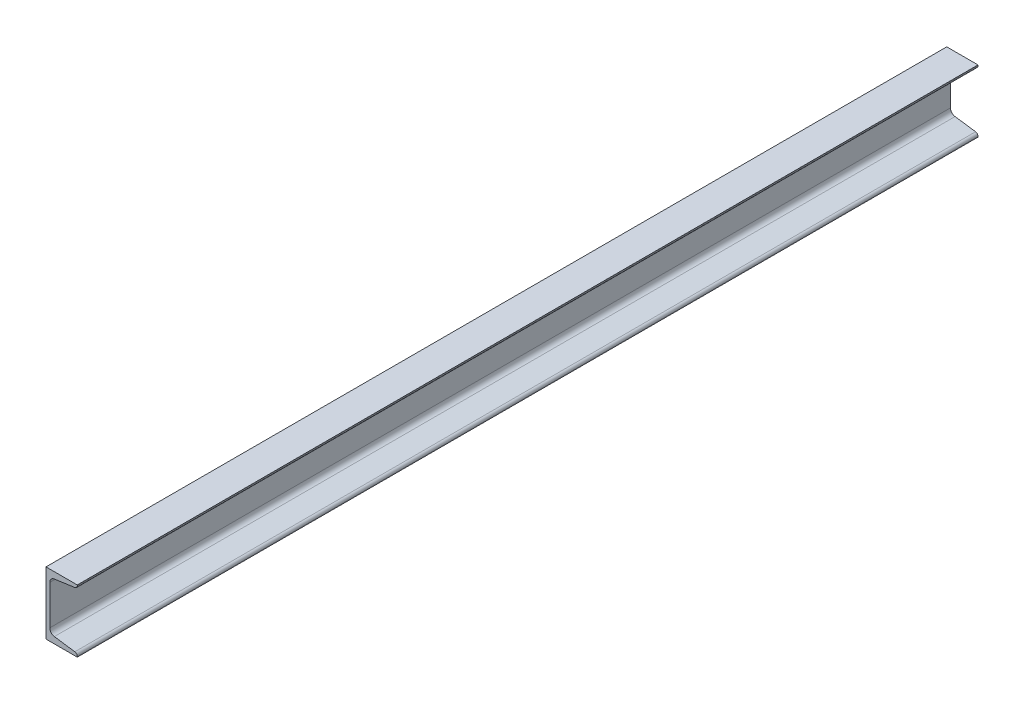
from build123d import *

# Parameters (mm, degrees)
BOSS_EXTRUDE1_DEPTH = 1440
SKETCH2_R           = 8.5
CUT_EXTRUDE1_DEPTH  = 1440


with BuildPart() as part:
    # Sketch1 → Boss-Extrude1 (new body)
    with BuildSketch(Plane.XY):
        with BuildLine():
            Line((0, 0), (-50, 0))
            Line((-50, 0), (-50, -100))
            Line((-50, -100), (0, -100))
            Line((0, -100), (0, -98.925311188))
            ThreePointArc((0, -98.925311188), (-1.103806889, -95.973045557), (-3.873721046, -94.469104878))
            Line((-3.873721046, -94.469104878), (-36.682971358, -89.858065454))
            ThreePointArc((-36.682971358, -89.858065454), (-41.915031432, -87.017288616), (-44, -81.440786869))
            Line((-44, -81.440786869), (-44, -18.559213131))
            ThreePointArc((-44, -18.559213131), (-41.915031432, -12.982711384), (-36.682971358, -10.141934546))
            Line((-36.682971358, -10.141934546), (-3.873721046, -5.530895122))
            ThreePointArc((-3.873721046, -5.530895122), (-1.103806889, -4.026954443), (0, -1.074688812))
            Line((0, -1.074688812), (0, 0))
        make_face()
    extrude(amount=BOSS_EXTRUDE1_DEPTH)

    # Sketch2 → Cut-Extrude1 (cut)
    with BuildSketch(Plane.ZY.offset(50)):
        with Locations(Location((73.2, -38, 0), (0, 0, 270))):
            Circle(SKETCH2_R)
        with Locations(Location((234.9, -38, 0), (0, 0, 270))):
            Circle(SKETCH2_R)
        with Locations(Location((396.6, -38, 0), (0, 0, 270))):
            Circle(SKETCH2_R)
        with Locations(Location((558.3, -38, 0), (0, 0, 270))):
            Circle(SKETCH2_R)
        with Locations(Location((720, -38, 0), (0, 0, 270))):
            Circle(SKETCH2_R)
        with Locations(Location((881.7, -38, 0), (0, 0, 270))):
            Circle(SKETCH2_R)
        with Locations(Location((1043.4, -38, 0), (0, 0, 270))):
            Circle(SKETCH2_R)
        with Locations(Location((1205.1, -38, 0), (0, 0, 270))):
            Circle(SKETCH2_R)
        with Locations(Location((1366.8, -38, 0), (0, 0, 270))):
            Circle(SKETCH2_R)
    extrude(amount=-CUT_EXTRUDE1_DEPTH, mode=Mode.SUBTRACT)


solid = part.part
